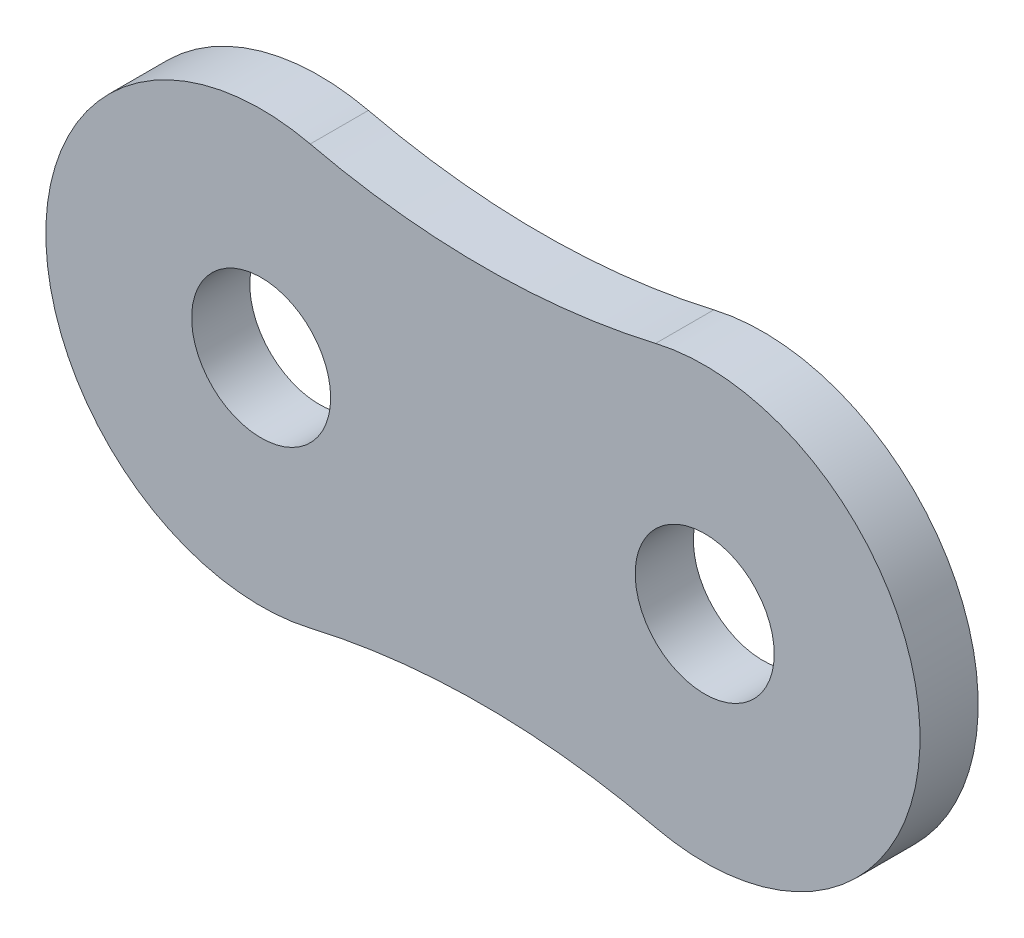
from build123d import *

# Parameters (mm, degrees)
EXTRUDE_1_DEPTH     = 1.665
SKETCH_3_R          = 1.99
CUT_EXTRUDE_1_DEPTH = 15.050077402


with BuildPart() as part:
    # 草图2 → 拉伸1 (new body)
    with BuildSketch(Plane.XY):
        with BuildLine():
            ThreePointArc((-4.944493019, 6.002647343), (-12.515, 0), (-4.944493019, -6.002647343))
            ThreePointArc((-4.944493019, -6.002647343), (0, -5.4315), (4.944493019, -6.002647343))
            ThreePointArc((4.944493019, -6.002647343), (12.515, 0), (4.944493019, 6.002647343))
            ThreePointArc((4.944493019, 6.002647343), (0, 5.4315), (-4.944493019, 6.002647343))
        make_face()
    extrude(amount=EXTRUDE_1_DEPTH)

    # 草图3 → 切除-拉伸1 (cut, through all)
    with BuildSketch(Plane.XY.offset(1.665)):
        with Locations((-6.35, 0)):
            Circle(SKETCH_3_R)
        with Locations((6.35, 0)):
            Circle(SKETCH_3_R)
    extrude(amount=-CUT_EXTRUDE_1_DEPTH, mode=Mode.SUBTRACT)


solid = part.part
